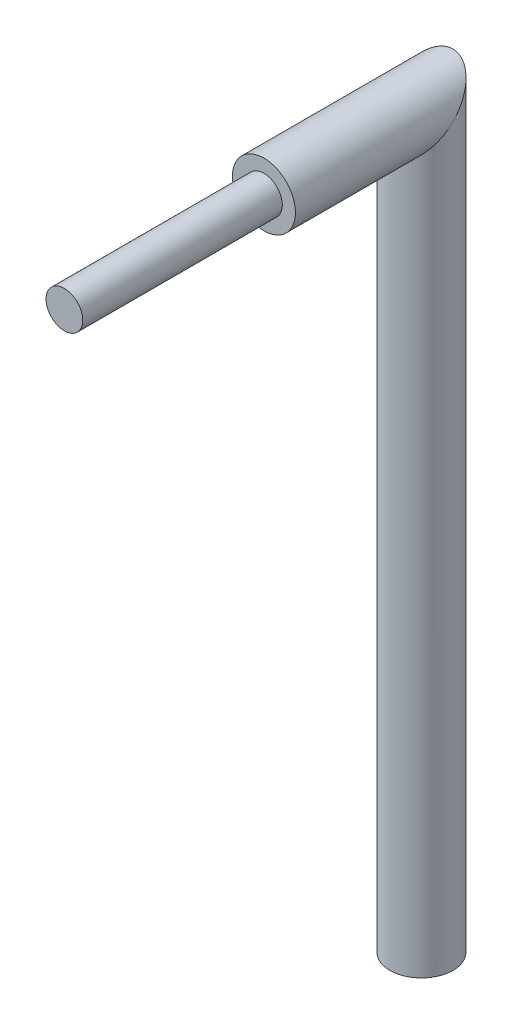
from build123d import *

# Parameters (mm, degrees)
SKETCH1_R           = 3
BOSS_EXTRUDE1_DEPTH = 70
SKETCH3_R           = 3
BOSS_EXTRUDE3_DEPTH = 15
BOSS_EXTRUDE4_DEPTH = 4
CUT_EXTRUDE1_DEPTH  = 77.216796049
SKETCH6_R           = 1.75
BOSS_EXTRUDE5_DEPTH = 19


with BuildPart() as part:
    # Sketch1 → Boss-Extrude1 (new body)
    with BuildSketch(Plane(origin=(0, 0, 0), x_dir=(1, 0, 0), z_dir=(0, 1, 0))):
        with Locations(Location((0, 0, 0), (0, 0, 270))):
            Circle(SKETCH1_R)
    extrude(amount=BOSS_EXTRUDE1_DEPTH)

    # Sketch3 → Boss-Extrude3 (add)
    with BuildSketch(Plane.XY):
        with Locations((0, 70)):
            Circle(SKETCH3_R)
    extrude(amount=BOSS_EXTRUDE3_DEPTH)

    # Sketch4 → Boss-Extrude4 (add)
    with BuildSketch(Plane(origin=(0, 70, 0), x_dir=(1, 0, 0), z_dir=(0, 1, 0))):
        with BuildLine():
            Line((-3, 0), (3, 0))
            ThreePointArc((3, 0), (0, 3), (-3, 0))
        make_face()
    extrude(amount=BOSS_EXTRUDE4_DEPTH)

    # Sketch5 → Cut-Extrude1 (cut, through all)
    with BuildSketch(Plane.XY.offset(15)):
        with BuildLine():
            Line((-3, 70), (-3, 74))
            Line((-3, 74), (3, 74))
            Line((3, 74), (3, 70))
            ThreePointArc((3, 70), (0, 73), (-3, 70))
        make_face()
    extrude(amount=-CUT_EXTRUDE1_DEPTH, mode=Mode.SUBTRACT)

    # Sketch6 → Boss-Extrude5 (add)
    with BuildSketch(Plane.XY.offset(15)):
        with Locations(Location((0, 70, 0), (0, 0, 180))):
            Circle(SKETCH6_R)
    extrude(amount=BOSS_EXTRUDE5_DEPTH)


solid = part.part
